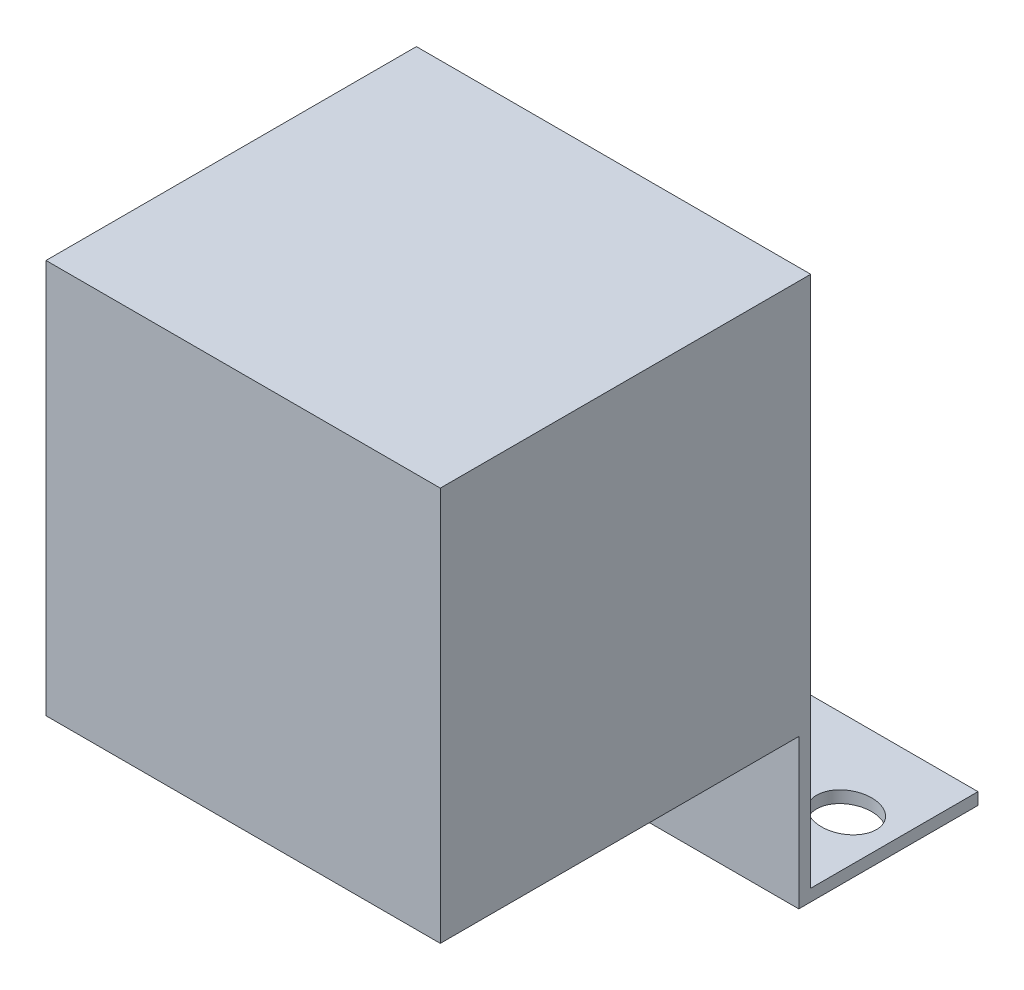
from build123d import *

# Parameters (mm, degrees)
SKETCH1_W          = 33
SKETCH1_H          = 33
EXTRUDE1_DEPTH     = 30
EXTRUDE2_DEPTH     = 16.5
SKETCH4_RX         = 2.5
SKETCH4_RY         = 2.1
CUT_EXTRUDE1_DEPTH = 57.147128155


with BuildPart() as part:
    # Sketch1 → Extrude1 (new body)
    with BuildSketch(Plane.XY):
        Rectangle(SKETCH1_W, SKETCH1_H)
    extrude(amount=EXTRUDE1_DEPTH)

    # Sketch3 → Extrude2 (add, symmetric)
    with BuildSketch(Plane(origin=(0, 0, 0), x_dir=(0, 0, -1), z_dir=(1, 0, 0))):
        Polygon((0, 16.5), (0, -29), (15, -29), (15, -28), (1, -28), (1, 16.5), align=None)
    extrude(amount=EXTRUDE2_DEPTH, both=True)

    # Sketch4 → Cut-Extrude1 (cut, through all)
    with BuildSketch(Plane(origin=(0, -28, 0), x_dir=(1, 0, 0), z_dir=(0, 1, 0))):
        with Locations(Location((-12.5, 8), (0, 0, 90))):
            Ellipse(SKETCH4_RX, SKETCH4_RY)
        with Locations(Location((12.5, 8), (0, 0, -180))):
            Ellipse(SKETCH4_RX, SKETCH4_RY)
    extrude(amount=-CUT_EXTRUDE1_DEPTH, mode=Mode.SUBTRACT)


solid = part.part
